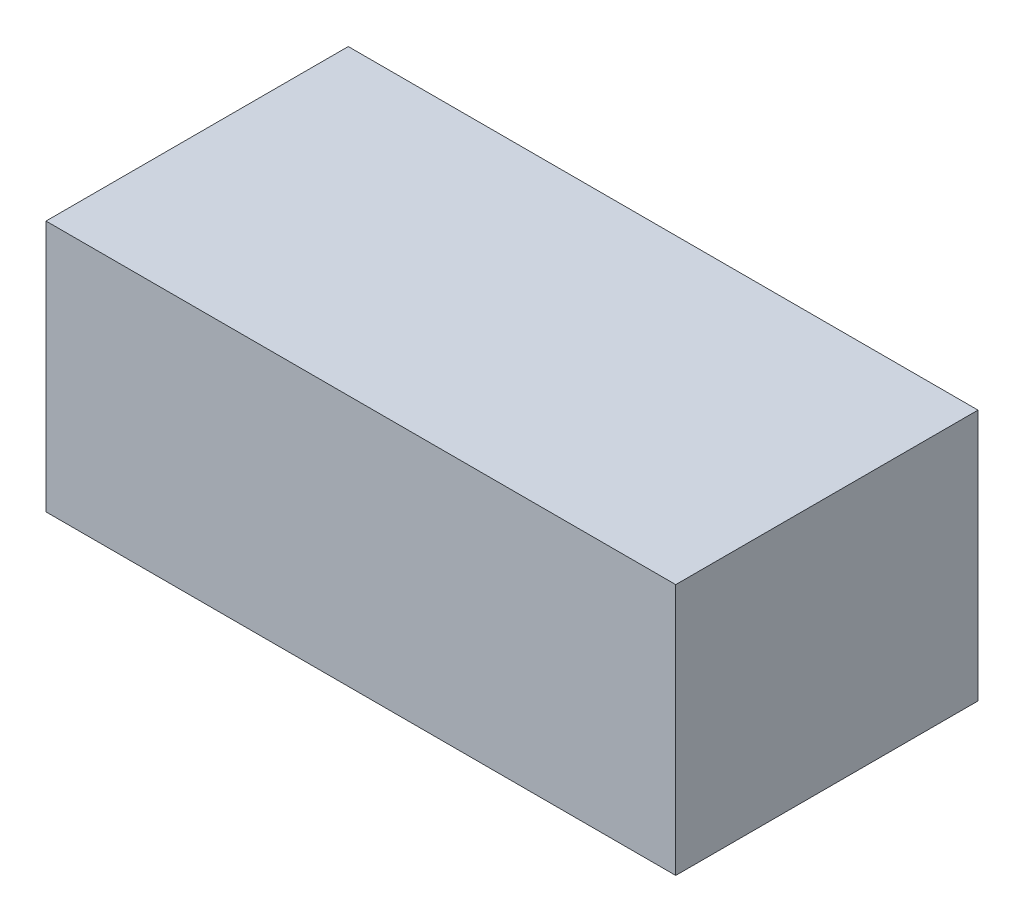
SolidWorks part; units mm, degrees
ref_plane "前视基准面" through (0, 0, 0) normal (0, 0, 1) x (1, 0, 0)
ref_plane "上视基准面" through (0, 0, 0) normal (0, 1, 0) x (1, 0, 0)
ref_plane "右视基准面" through (0, 0, 0) normal (1, 0, 0) x (0, 0, -1)
other "Configuration Table"
sketch "草图1" plane through (0, 0, 0) normal (0, 0, 1) x (1, 0, 0)
  line L0 (-12.5, -5) -> (12.5, -5)
  line L1 (12.5, -5) -> (12.5, 5)
  line L2 (12.5, 5) -> (-12.5, 5)
  line L3 (-12.5, 5) -> (-12.5, -5)
  point P0 (0, 0)
  dimension "D1" = 12.5
  dimension "D2" = 25
  dimension "D3" = 5
  dimension "D4" = 10
extrude "凸台-拉伸1" add sketch "草图1" against normal mid plane 12
